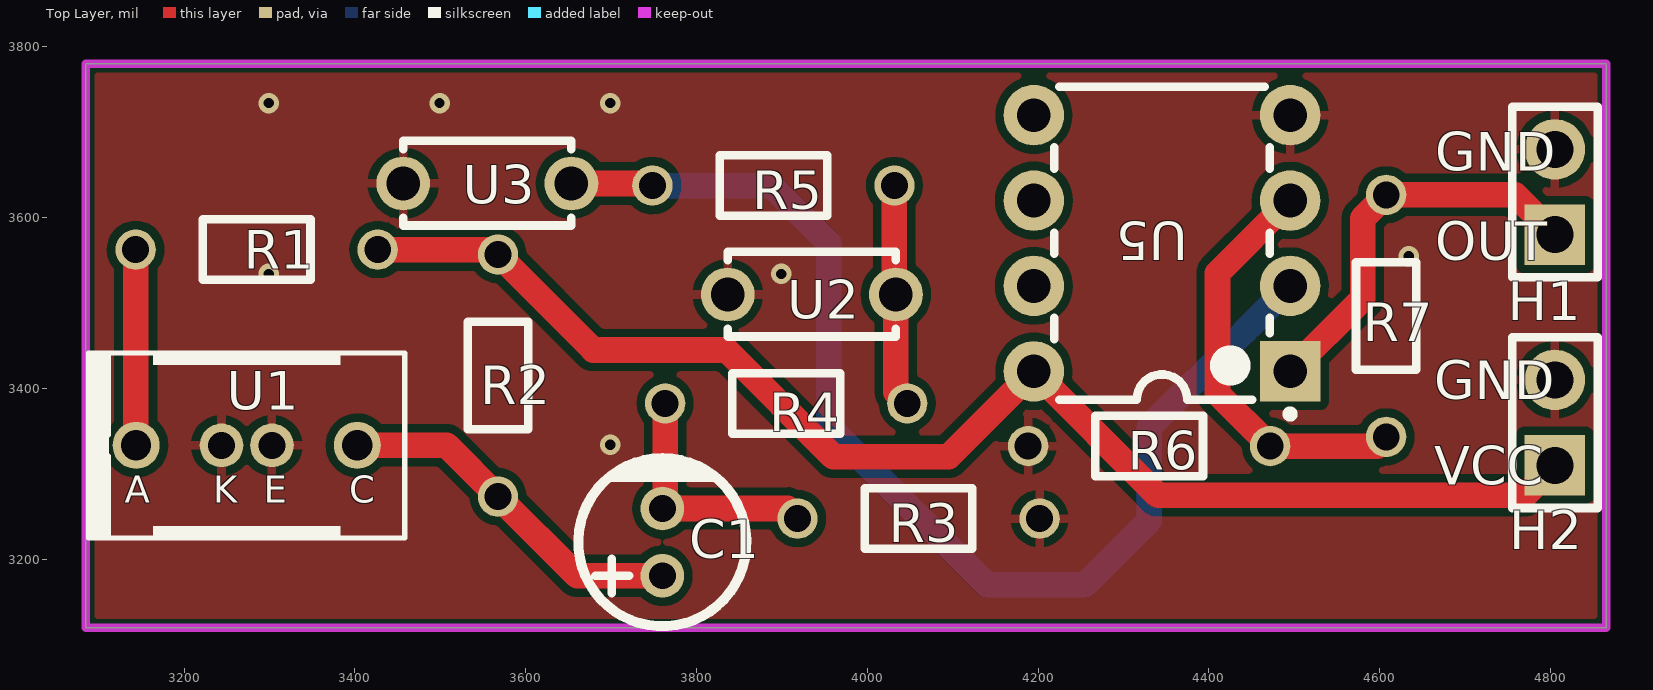
[diagram p0: Top Layer view]
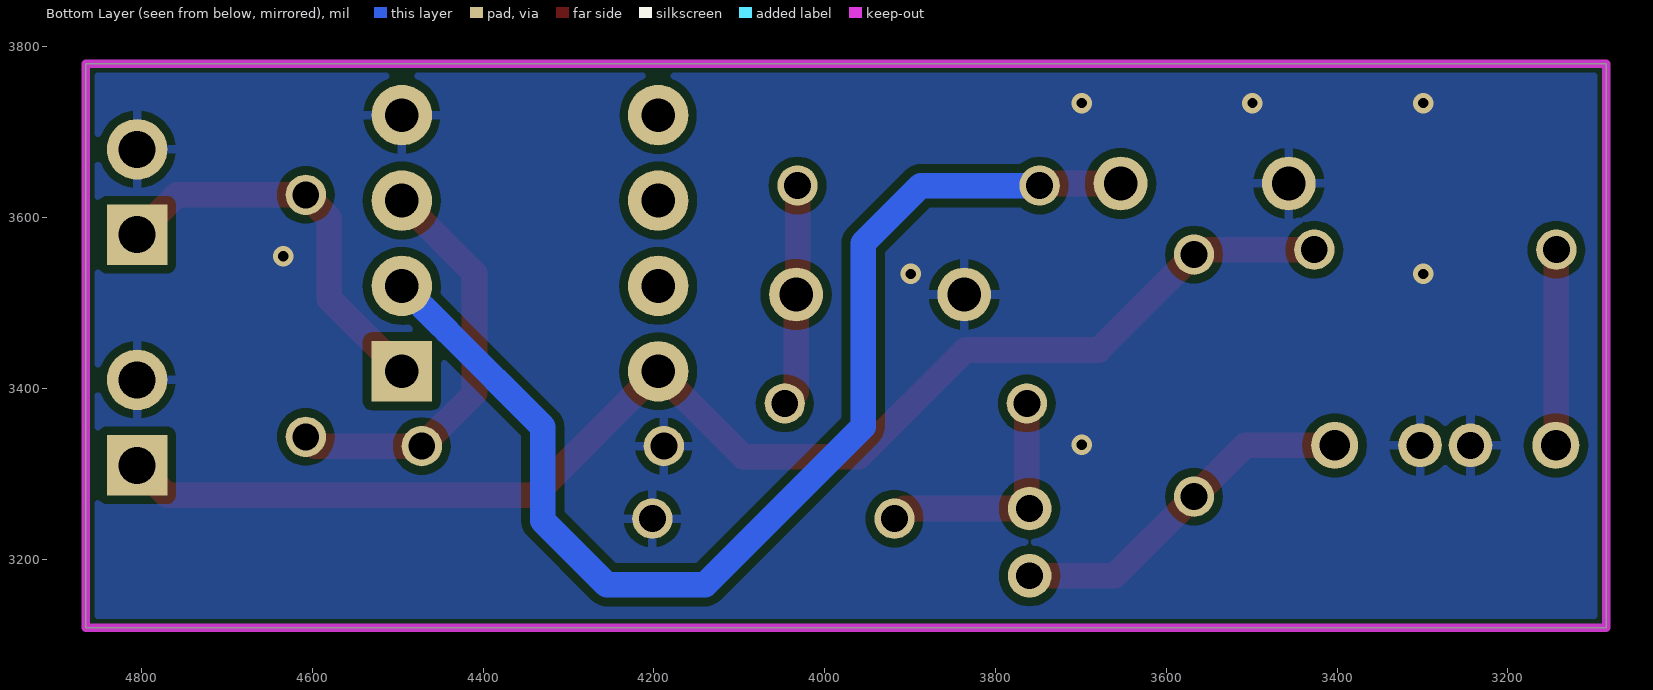
[diagram p1: Bottom Layer view, seen from below]
# Altium PCB MISC51900.pcbdoc
Units mil, origin at the board's own origin, x right, y up, seen from the top; angles counter-clockwise.
Board outline 1780 x 660 mil, 2 copper layers (Top Layer, Bottom Layer), stack 62.206 mil thick; 14 components, 9 nets, 36 pads, 7 vias.

## Layer stack, top to bottom
Top Solder Mask Layer: solder mask 0.394, Dk 3.3
Top Layer: signal copper 1.379
Dielectric1: surface 59.449, FR4, Dk 4.5
Bottom Layer: signal copper 1.378
Bottom Solder Mask Layer: solder mask 0.394, Dk 3.3

## Board outline
3085,3780 3085,3120 4865,3120 4865,3780

## Design rules (kind name [scope] priority, off if disabled: settings)
BoardOutlineClearance copperThickness2oz_1 [All] p2 off: genericclearance=7.99 ignorepadtopadclearanceinfootprint=FALSE except(0: Arc-SplitContinuation Track-SplitContinuation SMDPad-SplitContinuation THPad-SplitContinuation Via-SplitContinuation Fill-SplitContinuation Region-SplitContinuation Poly-SplitContinuation Text-SplitContinuation Hole-SplitContinuation; 5.98: Arc-CutoutEdge SMDPad-CutoutEdge THPad-CutoutEdge Via-CutoutEdge Fill-CutoutEdge Region-CutoutEdge Text-CutoutEdge; 6.93: Hole-OutlineEdge Hole-CutoutEdge; 10: Poly-OutlineEdge Poly-CutoutEdge; 11.81: Arc-OutlineEdge Track-OutlineEdge SMDPad-OutlineEdge THPad-OutlineEdge Via-OutlineEdge Fill-OutlineEdge Region-OutlineEdge Text-OutlineEdge Track-CutoutEdge)
BoardOutlineClearance copperThickness1oz_1 [All] p4: genericclearance=4.02 ignorepadtopadclearanceinfootprint=FALSE except(0: Arc-SplitContinuation Track-SplitContinuation SMDPad-SplitContinuation THPad-SplitContinuation Via-SplitContinuation Fill-SplitContinuation Region-SplitContinuation Poly-SplitContinuation Text-SplitContinuation Hole-SplitContinuation; 6: SMDPad-CutoutEdge THPad-CutoutEdge Via-CutoutEdge Fill-CutoutEdge Region-CutoutEdge Text-CutoutEdge; 6.93: Hole-OutlineEdge Hole-CutoutEdge; 10: Poly-OutlineEdge Poly-CutoutEdge; 11.8: Arc-OutlineEdge Track-OutlineEdge SMDPad-OutlineEdge THPad-OutlineEdge Via-OutlineEdge Fill-OutlineEdge Region-OutlineEdge Text-OutlineEdge; 11.81: Arc-CutoutEdge Track-CutoutEdge)
Clearance copperThickness2oz [All] p1 off: gap=7.99 ignorepadtopadclearanceinfootprint=FALSE except(5.98: SMDPad-Track SMDPad-SMDPad THPad-Track SMDPad-THPad THPad-THPad Track-Via SMDPad-Via THPad-Via Via-Via Fill-Track Region-Track Fill-SMDPad Region-SMDPad Fill-THPad Region-THPad Fill-Via Region-Via Fill-Fill Fill-Region Region-Region Arc-Track Arc-SMDPad Arc-THPad Arc-Via Fill-Arc Region-Arc Arc-Arc Text-Track SMDPad-Text Text-THPad Text-Via Fill-Text Region-Text Arc-Text Text-Text; 6.93: Hole-Track Hole-SMDPad Hole-THPad Hole-Via Fill-Hole Region-Hole Hole-Arc Hole-Text; 10: Poly-Track Poly-SMDPad Poly-THPad Poly-Via Poly-Fill Poly-Region Poly-Poly Poly-Arc Poly-Text Poly-Hole)
Clearance copperThickness1oz [All] p3: gap=4.02 ignorepadtopadclearanceinfootprint=FALSE except(5.98: SMDPad-Track SMDPad-SMDPad THPad-Track SMDPad-THPad THPad-THPad Track-Via SMDPad-Via THPad-Via Via-Via Fill-Track Region-Track Fill-SMDPad Region-SMDPad Fill-THPad Region-THPad Fill-Via Region-Via Fill-Fill Fill-Region Region-Region; 6: Arc-Track Arc-SMDPad Arc-THPad Arc-Via Fill-Arc Region-Arc Arc-Arc Text-Track SMDPad-Text Text-THPad Text-Via Fill-Text Region-Text Arc-Text Text-Text; 6.93: Hole-Track Hole-SMDPad Hole-THPad Hole-Via Fill-Hole Region-Hole Hole-Arc Hole-Text; 10: Poly-Track Poly-SMDPad Poly-THPad Poly-Via Poly-Fill Poly-Region Poly-Poly Poly-Arc Poly-Text Poly-Hole)
DiffPairsRouting differentialPair [All] p1: maxlimit=6 minlimit=6 mostfreqgap=6 toplayer_minwidth=5 toplayer_prefwidth=10 toplayer_maxwidth=100 toplayer_mingap=6 toplayer_prefgap=6 toplayer_maxgap=6 bottomlayer_minwidth=5 bottomlayer_prefwidth=10 bottomlayer_maxwidth=100 bottomlayer_mingap=6 bottomlayer_prefgap=6 bottomlayer_maxgap=6 maxuncoupledlength=10
HoleToHoleClearance otherClearance [All] p1: gap=11.81 allowstackedmicrovias=TRUE
Length netLength [All] p1: minlimit=0 maxlimit=0
MatchedLengths netLengthTolerance [All] p1: tolerance=1000
PasteMaskExpansion pasteMaskExpansion [All] p1: expansion=0
PlaneConnect innerPlane [All] p1: planeconnectstyle=Relief reliefexpansion=20 reliefentries=4 reliefconductorwidth=10 reliefairgap=10
PolygonConnect copperRegion [(InNet('GND'))] p1: connectstyle=Relief reliefconductorwidth=10 reliefentries=4 polygonreliefangle="90 Angle" airgapwidth=10 via.connectstyle=Relief via.reliefconductorwidth=10 via.reliefentries=4 via.polygonreliefangle="90 Angle" via.airgapwidth=10
RoutingVias viaSize [All] p1: holewidth=12.01 width=24.02 viastyle="Through Hole" minholewidth=11.81 minwidth=19.68 maxholewidth=248.03 maxwidth=393.7
SolderMaskExpansion solderMaskExpansion [IsVia] p1: expansion=-1000 istentingtop=TRUE
SolderMaskExpansion solderMaskExpansion [All] p2: expansion=2 istentingtop=FALSE
Width copperThickness2oz_2 [All] p1 off: maxlimit=100 minlimit=8 preferedwidth=10
Width copperThickness1oz_2 [All] p2: maxlimit=100 minlimit=5 preferedwidth=10

## Components (designator, comment, footprint, x,y, rotation, side; value= is the part's Value field where it differs from the comment)
C1 "10uF" CAP-TH_BD5.0-P2.00-D0.8-FD-10UF50VC110GL 3760,3220 r90 top
H1 "" HDR-TH_2P-P2.54-V-M-1 4805,3630 r90 top
H2 "" HDR-TH_2P-P2.54-V-M-1 4805,3360 r90 top
R1 "560Ω" Res_1/8W 3285,3560 r0 top
R2 "560Ω" Res_1/8W 3570,3415 r90 top
R3 "20KΩ" Res_1/8W 4060,3250 r180 top
R4 "10kΩ" Res_1/8W 3905,3380 r0 top
R5 "10kΩ" Res_1/8W 3890,3640 r180 top
R6 "220Ω" Res_1/8W 4330,3330 r0 top
R7 "120kΩ" Res_1/8W 4610,3485 r90 top
U1 "ST188" OPTO-TH_ST188 3273.32,3333.33 r0 top
U2 "105" CAP-TH_L5.0-W2.5-P5.00-D1.0 3935,3510 r180 top
U3 "105" CAP-TH_L5.0-W2.5-P5.00-D1.0 3555,3640 r180 top
U5 "LM358N" DIP-8_L9.2-W6.4-P2.54-LS7.6-BL 4345,3570 r90 top

## Footprints (in the part's own frame and the unit in brackets; to place one, negate y for a bottom-side part, rotate by r counter-clockwise, add the part's x,y. Pads: shape width x height; smd on the part's side, far side on the other; paste and mask are expansions set on the pad)
CAP-TH_BD5.0-P2.00-D0.8-FD-10UF50VC110GL [mm]
  round 1.3 hole 0.8: 1(-1,0) 2(1,0)
  silkscreen extent -2.5,-2.5 2.5,2.5
CAP-TH_L5.0-W2.5-P5.00-D1.0 [mm]
  round 1.6 hole 1: 1(-2.5,0) 2(2.5,0)
  silkscreen extent -2.5,-1.27 2.5,1.25
DIP-8_L9.2-W6.4-P2.54-LS7.6-BL [mm]
  rect 1.8x1.8 hole 1: 1(-3.81,-3.81)
  round 1.8 hole 1: 2(-1.27,-3.81) 3(1.27,-3.81) 4(3.81,-3.81) 5(3.81,3.81) 6(1.27,3.81) 7(-1.27,3.81) 8(-3.81,3.81)
  silkscreen extent -5.18,-3.91 4.65,3.2
HDR-TH_2P-P2.54-V-M-1 [mm]
  rect 1.8x1.8 hole 1.1: 1(-1.27,0)
  round 1.8 hole 1.1: 2(1.27,0)
  silkscreen extent -2.54,-1.27 2.54,1.27
OPTO-TH_ST188 [mm]
  round 1.4 hole 0.9 paste+0 mask+0.05: 1(-3.29,0) 4(3.29,0)
  round 1.3 hole 0.8 paste+0 mask+0.05: 2(-0.75,0) 3(0.75,0)
  silkscreen extent -4.7,-2.75 4.7,2.75
Res_1/8W [mil]
  round 47.2 hole 31.5 paste+0 mask+2: 1(-141.7,2.48) 2(141.7,2.48)
  silkscreen extent -63,-33 63,38

## Via types
v1: diameter 24.02, hole 12, Top Layer to Bottom Layer, 7 vias

## Nets (pads, with @x,y where several pads share a name; then routed paths per layer and width w, separated by ;. In a path a pad name is that pad's centre, name@x,y a point inside that pad or via, vN(x,y) a via of type N, cw(c..) or ccw(c..) an arc to the next point about the centre after c; other vN are vias at no path point)
$1N2: R1.1 U1.1 | length 229.4
  Top Layer w30: R1.1 3143.3,3333.81 U1.1
$1N4: C1.1 R2.1 U1.4 | length 420.4
  Top Layer w30: U1.4 3507.5,3333.32 R2.1 3660.19,3180.63 C1.1
$1N7: C1.2 R3.2 R4.1 | length 287.7
  Top Layer w30: R4.1 3763.3,3262.67 C1.2 3906.45,3259.37 R3.2
$1N9: R4.2 R5.1 U2.1 | length 261.3
  Top Layer w30: R5.1 4031.7,3511.72 U2.1 4033.43,3395.75 R4.2
$1N12: R5.2 U3.1 U5.2 | length 1371.7
  Top Layer w30: U3.1 3745.82,3640 R5.2
  Bottom Layer w30: R5.2 3887.48,3637.52 3955,3570 3955,3355 4140,3170 4255,3170 4330,3245 4330,3355 4442.18,3467.18 cw(c4459.57,3455.43) 4447.82,3472.82 U5.2
$1N18: R6.2 R7.1 U5.3 | length 488.6
  Top Layer w30: U5.3 4410,3535 4410,3394.18 R6.2 4596.7,3332.48 R7.1
GND: H1.2 H2.2 R3.1 R6.1 U1.2 U1.3 U2.2 U3.2 U5.4
  other v1: 3699.1,3334.1 3299.1,3534.1 3899.1,3534.1 4633.91,3554.88 3299.1,3734.1 3499.1,3734.1 3699.1,3734.1
OUT: H1.1 R7.2 U5.1 | length 470.1
  Top Layer w30: U5.1 4580,3505 4580,3599.18 R7.2 4758.3,3626.7 H1.1
VCC: H2.1 R1.2 R2.2 U5.8 | length 1594.7
  Top Layer w30: R1.2 3561.75,3562.48 R2.2 3679.22,3445 3835,3445 3960,3320 4095,3320 U5.8 4340,3275 4770,3275 H2.1
pads on no net: U5.5 U5.6 U5.7

## Polygon pours and split planes (outlines as drawn)
GND on Bottom Layer (solid, remove dead copper, pour order 2): 3000,3880 3000,3000 4930,3000 4930,3880
GND on Top Layer (solid, remove dead copper, pour order 0): 3030,3850 3030,3020 5000,3020 5000,3850

## Keep-outs
Board Outline Layer:
  the board outline again, w10

## Silkscreen, mask and mechanical layers (free items; w line width, h text height)
Top Silkscreen Layer:
  text "GND" at 4665,3655 h45
  text "OUT" at 4665,3550 h45
  text "GND" at 4663.95,3387.5 h45
  text "VCC" at 4663.95,3287.5 h45